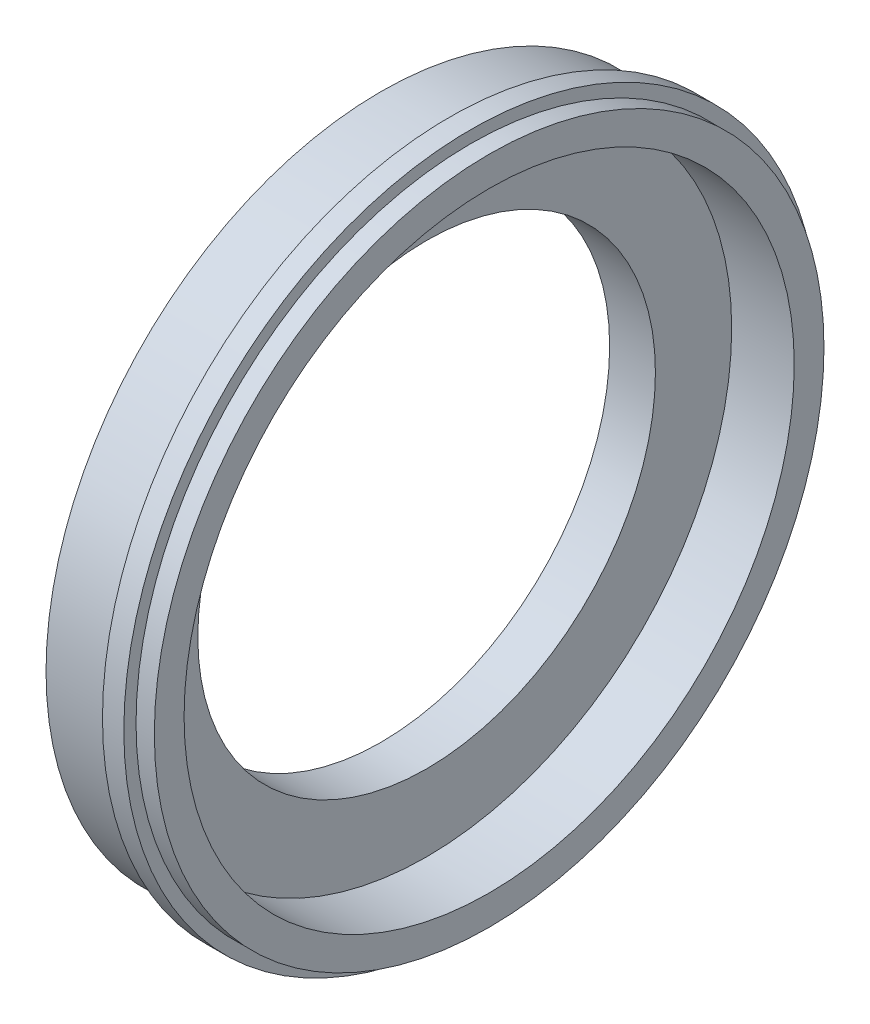
SolidWorks part; units mm, degrees
material "灰铸铁 HT150 "
ref_plane "Front Plane" through (0, 0, 0) normal (0, 0, 1) x (1, 0, 0)
ref_plane "Top Plane" through (0, 0, 0) normal (0, 1, 0) x (1, 0, 0)
ref_plane "Right Plane" through (0, 0, 0) normal (1, 0, 0) x (0, 0, -1)
sketch "Sketch1" plane through (0, 0, 0) normal (0, 1, 0) x (1, 0, 0)
  line L0 (0, 0) -> (212.6126, 0) construction
  line L1 (0, 150) -> (0, 163)
  line L2 (0, 219.5) -> (45, 219.5)
  line L3 (45, 219.5) -> (45, 227.5)
  line L4 (45, 227.5) -> (59, 227.5)
  line L5 (59, 227.5) -> (59, 219.5)
  line L6 (59, 219.5) -> (71, 219.5)
  line L7 (71, 219.5) -> (71, 200)
  line L8 (71, 200) -> (30, 200)
  line L9 (30, 200) -> (30, 150)
  line L10 (30, 150) -> (0, 150)
  line L15 (0, 203) -> (0, 219.5)
  line L16 (0, 203) -> (14, 203)
  line L17 (0, 189) -> (14, 189)
  line L18 (14, 203) -> (14, 189)
  line L19 (0, 177) -> (0, 189)
  line L20 (0, 177) -> (14, 177)
  line L21 (0, 163) -> (14, 163)
  line L22 (14, 177) -> (14, 163)
  dimension "D1" = 150
  dimension "D2" = 163
  dimension "D3" = 177
  dimension "D4" = 189
  dimension "D5" = 203
  dimension "D6" = 219.5
  dimension "D7" = 14
  dimension "D8" = 227.5
  dimension "D9" = 14
  dimension "D10" = 26
  dimension "D11" = 71
  dimension "D12" = 200
  dimension "D13" = 30
revolve "Revolve1" add sketch "Sketch1" angle 360 about L0
